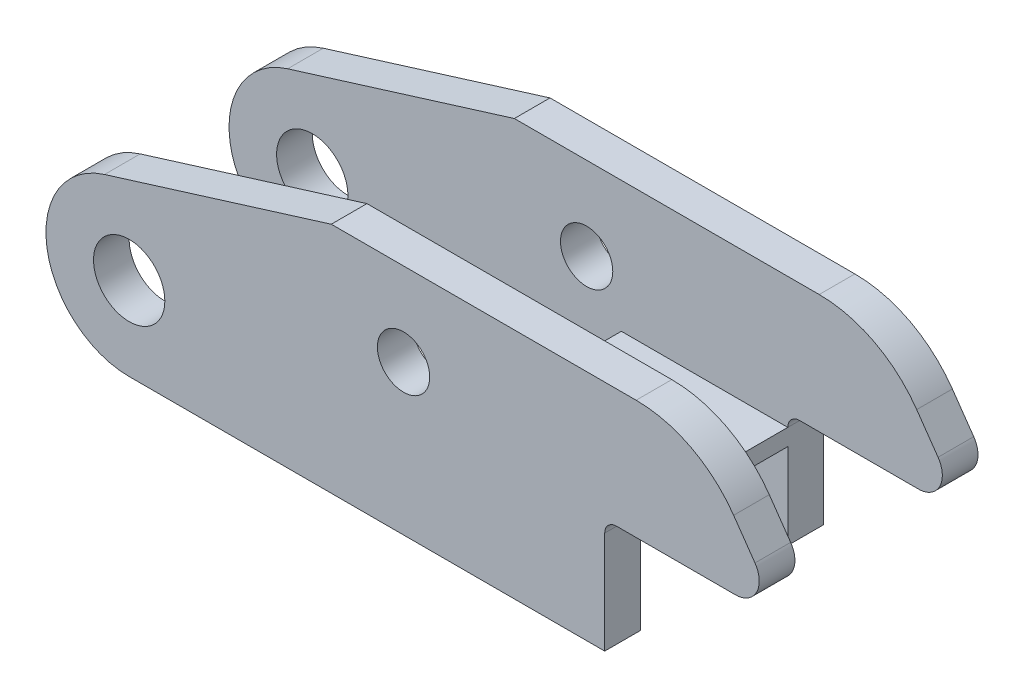
SolidWorks part; units mm, degrees
material "Q235铸造"
ref_plane "前视基准面" through (0, 0, 0) normal (0, 0, 1) x (1, 0, 0)
ref_plane "上视基准面" through (0, 0, 0) normal (0, 1, 0) x (1, 0, 0)
ref_plane "右视基准面" through (0, 0, 0) normal (1, 0, 0) x (0, 0, -1)
sketch "草图1" plane through (0, 0, -2290.8279) normal (0, 0, 1) x (1, 0, 0)
  line L0 (4, 81) -> (-196, 81)
  line L1 (4, 124) -> (4, 54) construction
  line L2 (17.2094, 179) -> (-111, 179)
  line L3 (58.224, 157.5972) -> (67.2029, 144.7194)
  line L4 (79, 129) -> (9, 129) construction
  line L5 (59, 129) -> (4, 129)
  line L6 (4, 129) -> (4, 81)
  line L7 (-111, 179) -> (-206.3656, 149.4298)
  line L8 (69, 139) -> (69, 201.8882) construction
  line L9 (84, 54) -> (84, 124) construction
  arc A0 (17.2094, 179) -> (58.224, 157.5972) centre (17.2094, 129) cw
  arc A1 (59, 129) -> (67.2029, 144.7194) centre (59, 139) ccw
  arc A2 (-206.3656, 149.4298) -> (-196, 81) centre (-196, 116) ccw
  circle A3 centre (-196, 116) radius 15
  point P14 (78.1632, 129)
  dimension "D3" = 50
  dimension "D4" = 10
  dimension "D5" = 70
  dimension "D2" = 30
  dimension "D9" = 15
  dimension "D1" = 200
  dimension "D6" = 98
  dimension "D7" = 50
  dimension "D8" = 180
extrude "凸台-拉伸1" add sketch "草图1" along normal blind 15 from offset 700
pattern_linear "阵列(线性)1" count 2 spacing 77 along (0, 0, 1) of bodies 106
sketch "草图2" plane through (4, 0, 0) normal (-1, 0, 0) x (0, 0, 1)
  line L0 (-1575.8279, 81) -> (-1575.8279, 149.4298) construction
  line L1 (-1575.8279, 124) -> (-1513.8279, 124)
  line L2 (-1575.8279, 124) -> (-1575.8279, 117)
  line L3 (-1575.8279, 117) -> (-1513.8279, 117)
  line L4 (-1513.8279, 124) -> (-1513.8279, 117)
  line L5 (-2290.8279, 124) -> (-25.8279, 124) construction
  line L6 (-1513.8279, 149.4298) -> (-1513.8279, 81) construction
  dimension "D1" = 7
extrude "凸台-拉伸2" add sketch "草图2" along normal blind 70
sketch "草图3" plane through (0, 0, -1513.8279) normal (0, 0, -1) x (-1, 0, 0)
  line L0 (-17.2094, 179) -> (111, 179) construction
  circle A0 centre (80.6052, 144) radius 11
  arc A1 (196, 81) -> (206.3656, 149.4298) centre (196, 116) ccw construction
  point P4 (230.6052, 110.7581)
  dimension "D1" = 22
  dimension "D2" = 35
  dimension "D3" = 150
extrude "切除-拉伸2" cut sketch "草图3" against normal mid plane 210
fillet "圆角1" radius 5 2 edges at (4, 129, -1583.3279) (4, 129, -1506.3279)
